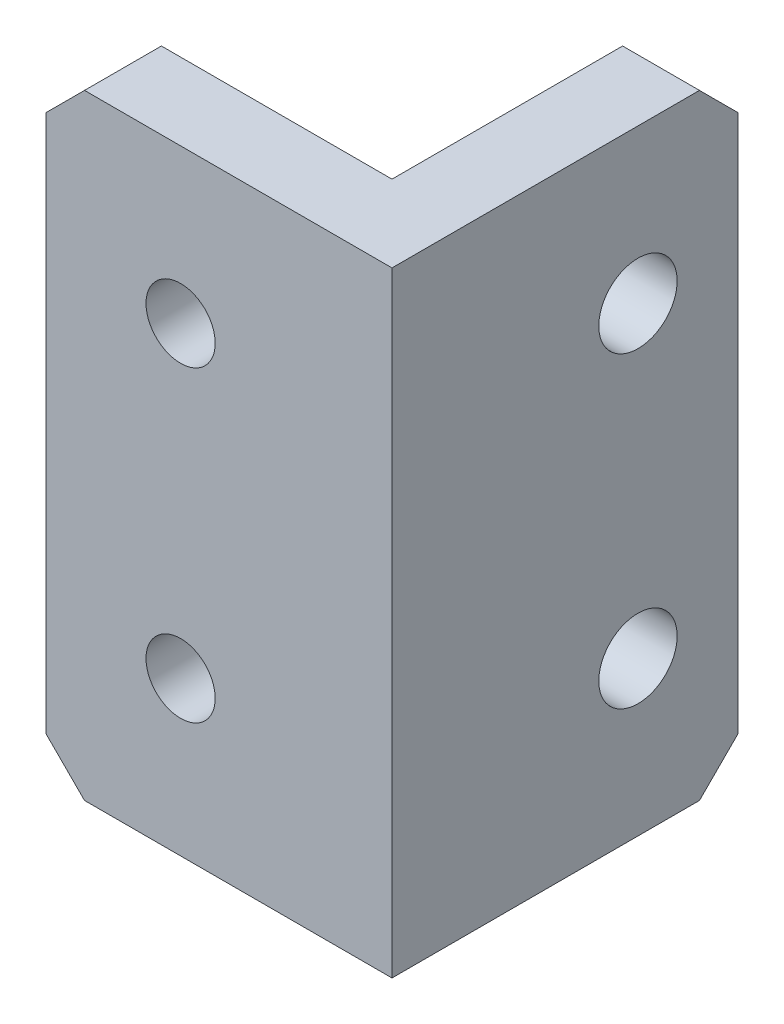
SolidWorks part; units mm, degrees
material "AISI 1045 钢，冷拔"
ref_plane "前视基准面" through (0, 0, 0) normal (0, 0, 1) x (1, 0, 0)
ref_plane "上视基准面" through (0, 0, 0) normal (0, 1, 0) x (1, 0, 0)
ref_plane "右视基准面" through (0, 0, 0) normal (1, 0, 0) x (0, 0, -1)
sketch "草图1" plane through (0, 0, 0) normal (0, 1, 0) x (1, 0, 0)
  line L0 (-22.5, -12.5) -> (12.5, -12.5)
  line L3 (-22.5, -22.5) -> (22.5, -22.5)
  line L4 (22.5, 22.5) -> (22.5, -22.5)
  line L5 (-22.5, 22.5) -> (22.5, -22.5) construction
  line L6 (-22.5, -22.5) -> (22.5, 22.5) construction
  line L7 (12.5, 22.5) -> (12.5, -12.5)
  line L8 (-22.5, -12.5) -> (-22.5, -22.5)
  line L9 (12.5, 22.5) -> (22.5, 22.5)
  point P0 (0, 0)
  dimension "D1" = 45
  dimension "D2" = 45
  dimension "D3" = 10
extrude "凸台-拉伸1" add sketch "草图1" along normal blind 80
chamfer "倒角1" distance 5 angle 45 4 edges at (17.5, 80, -22.5) (17.5, 0, -22.5) (-22.5, 0, 17.5) (-22.5, 80, 17.5)
sketch "草图2" plane through (0, 0, 12.5) normal (0, 0, -1) x (-1, 0, 0)
  line L0 (22.5, 40) -> (-30.3349, 40) construction
  line L1 (22.5, 75) -> (22.5, 5) construction
  line L2 (5, 60) -> (5, 20) construction
  dimension "D1" = 17.5
  dimension "D2" = 40
hole_wizard "M8 间隙孔1" positions "3D草图1" profile "草图3" hole size "M8" standard "GB"
sketch3d "3D草图1"
  point P0 (-5, 60, 12.5)
  point P3 (-5, 20, 12.5)
sketch "草图3" plane through (-5, 60, 12.5) normal (1, 0, 0) x (0, 1, 0)
  line L0 (0, 0) -> (0, 17.7039)
  line L1 (0, 17.7039) -> (4.5, 15)
  line L2 (4.5, 15) -> (4.5, 0)
  line L5 (4.5, 0) -> (0, 0)
  line L10 (0, 17.7039) -> (-4.5, 15) construction
  line L11 (0, -6.35) -> (0, 107.95) construction
  dimension "孔直径" = 9
  dimension "孔深度" = 15
  dimension "导头角度" = 118
sketch "草图4" plane through (12.5, 0, 0) normal (-1, 0, 0) x (0, 0, 1)
  line L0 (-9.5168, 86.3946) -> (-9.5168, -14.4244) construction
  line L1 (-22.5, 40) -> (7.435, 40) construction
  line L2 (-22.5, 75) -> (-22.5, 5) construction
  point P6 (-9.5168, 40)
hole_wizard "M12 螺纹孔1" positions "3D草图3" profile "草图7" tap size "M12" standard "GB" end condition through all
sketch3d "3D草图3"
  line L0 (12.5, 75, -22.5) -> (12.5, 5, -22.5) construction
  line L1 (12.5, 80, -17.5) -> (12.5, 80, 12.5) construction
  point P0 (12.5, 60, -9.5)
  dimension "D1" = 13
  dimension "D2" = 20
cosmetic thread "孔螺蚊线2" parameters "D2"=12
sketch "草图7" plane through (12.5, 60, -9.5) normal (0, 1, 0) x (0, 0, 1)
  line L0 (0, 0) -> (0, 10)
  line L1 (0, 10) -> (5.1, 10)
  line L2 (5.1, 10) -> (5.1, 0)
  line L5 (5.1, 0) -> (0, 0)
  line L11 (0, -6.35) -> (0, 107.95) construction
  dimension "通孔螺纹孔钻头直径" = 10.2
  dimension "通孔螺纹孔钻头深度" = 10
pattern_linear "阵列(线性)1" count 2 spacing 40 along (0, -1, 0) of "M12 螺纹孔1"
